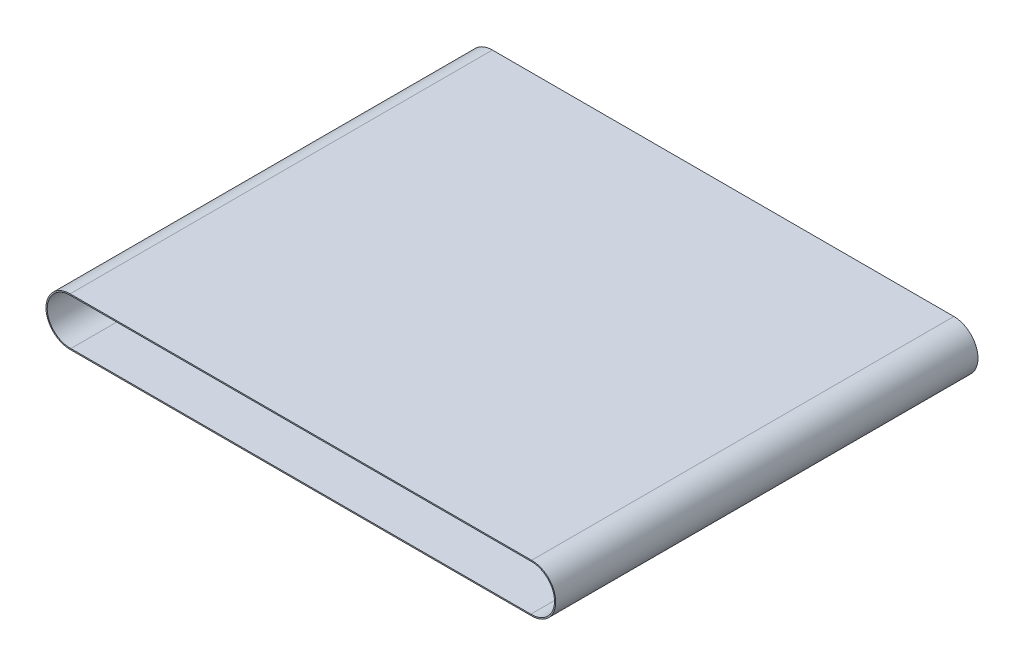
SolidWorks part; units mm, degrees
ref_plane "前视基准面" through (0, 0, 0) normal (0, 0, 1) x (1, 0, 0)
ref_plane "上视基准面" through (0, 0, 0) normal (0, 1, 0) x (1, 0, 0)
ref_plane "右视基准面" through (0, 0, 0) normal (1, 0, 0) x (0, 0, -1)
sketch "草图1" plane through (0, 0, 0) normal (0, 0, 1) x (1, 0, 0)
  line L0 (-382.5, 0) -> (0, 0) construction
  line L1 (0, 0) -> (382.5, 0) construction
  line L2 (-382.5, 0) -> (382.5, 0) construction
  line L3 (-382.5, 38) -> (382.5, 38)
  line L5 (0, 0) -> (0, -130.0789) construction
  line L9 (381.2663, -37.98) -> (-381.2663, -37.98)
  arc A0 (-382.5, 38) -> (-381.2663, -37.98) centre (-382.5, 0) ccw
  arc A1 (381.2663, -37.98) -> (382.5, 38) centre (382.5, 0) ccw
  point P3 (0, 0)
  dimension "D2" = 38
  dimension "D1" = 765
extrude "拉伸-薄壁1" add sketch "草图1" along normal mid plane 700 thin thin type one direction wall 2
sketch "草图4" plane through (0, 0, 0) normal (1, 0, 0) x (0, 0, -1)
  line L0 (0, 38) -> (0, 0) construction
  line L1 (-350, 38) -> (350, 38) construction
  line L2 (4, 38) -> (-4, 38)
  line L3 (-4, 38) -> (-2.5, 33)
  line L4 (-2.5, 33) -> (2.5, 33)
  line L5 (4, 38) -> (2.5, 33)
  line L6 (-350, 38) -> (350, 38) construction
  line L7 (0, 0) -> (0, 118.352) construction
  point P9 (0, 33)
  dimension "D1" = 8
  dimension "D2" = 5
extrude "凸台-拉伸2" add sketch "草图4" along normal blind 352 and the other way blind 361
